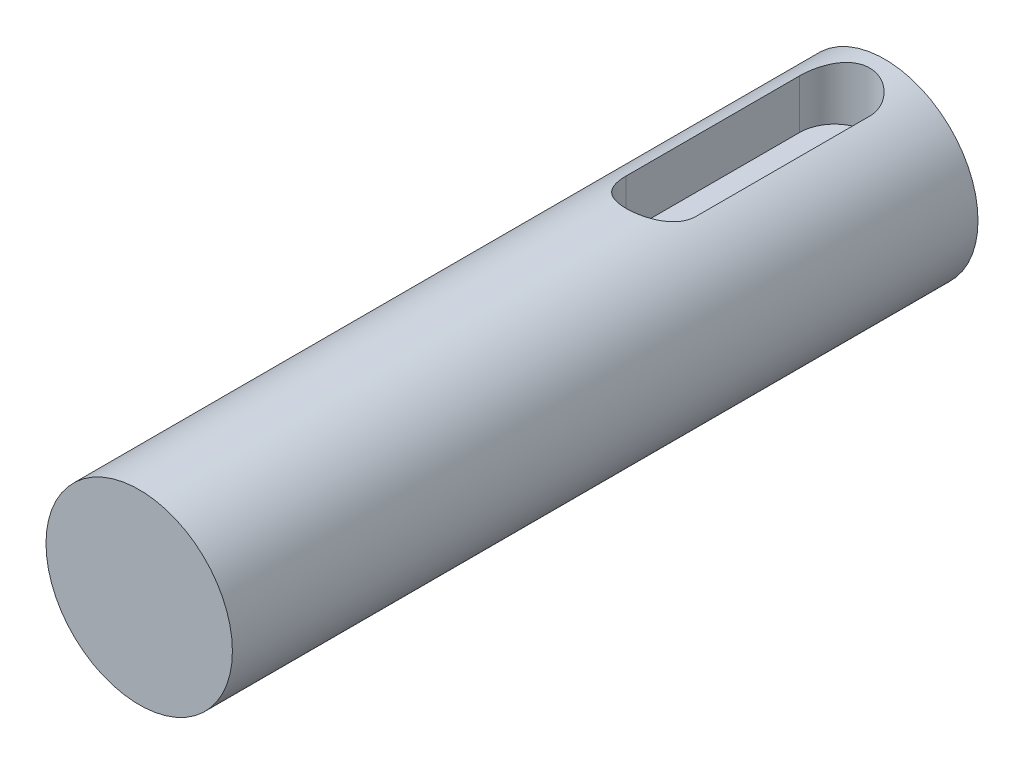
from build123d import *

# Parameters (mm, degrees)
SKETCH1_R           = 5
BOSS_EXTRUDE1_DEPTH = 40
CUT_EXTRUDE1_DEPTH  = 3


with BuildPart() as part:
    # Sketch1 → Boss-Extrude1 (new body)
    with BuildSketch(Plane.XY):
        Circle(SKETCH1_R)
    extrude(amount=BOSS_EXTRUDE1_DEPTH)

    # Sketch2 → Cut-Extrude1 (cut)
    with BuildSketch(Plane(origin=(0, 5, 0), x_dir=(1, 0, 0), z_dir=(0, 1, 0))):
        with BuildLine():
            Line((-1.876815102, -12), (-1.876815102, -2.691594063))
            ThreePointArc((-1.876815102, -2.691594063), (0, -0.814778961), (1.876815102, -2.691594063))
            Line((1.876815102, -2.691594063), (1.876815102, -12))
            ThreePointArc((1.876815102, -12), (0, -13.876815102), (-1.876815102, -12))
        make_face()
    extrude(amount=-CUT_EXTRUDE1_DEPTH, mode=Mode.SUBTRACT)


solid = part.part
